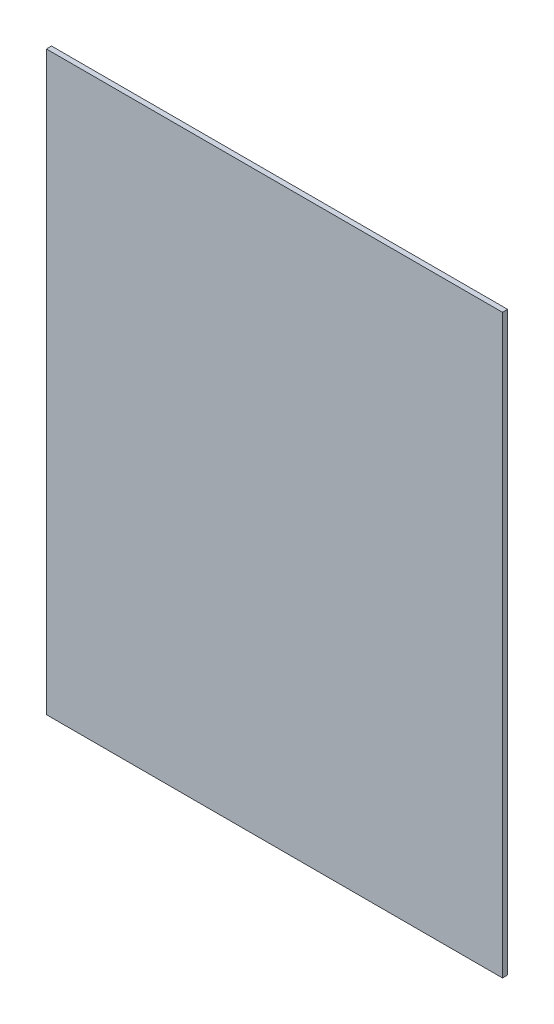
SolidWorks part; units mm, degrees
material "有机玻璃 (PMMA)"
ref_plane "前视" through (0, 0, 0) normal (0, 0, 1) x (1, 0, 0)
ref_plane "上视" through (0, 0, 0) normal (0, 1, 0) x (1, 0, 0)
ref_plane "右视" through (0, 0, 0) normal (1, 0, 0) x (0, 0, -1)
sketch "草图1" plane through (0, 0, 0) normal (0, 0, 1) x (1, 0, 0)
  line L1 (178, -225) -> (-178, -225)
  line L2 (178, -225) -> (178, 225)
  line L3 (178, 225) -> (-178, 225)
  line L4 (-178, -225) -> (-178, 225)
  line L5 (178, -225) -> (-178, 225) construction
  line L6 (178, 225) -> (-178, -225) construction
  point P0 (0, 0)
  dimension "D1" = 356
  dimension "D2" = 450
extrude "凸台-拉伸1" add sketch "草图1" along normal blind 4
